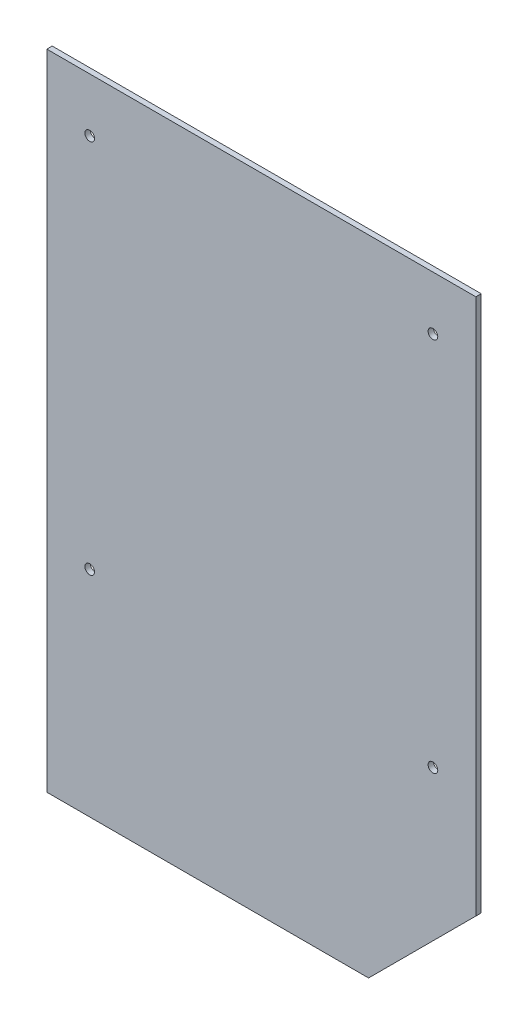
from build123d import *

# Parameters (mm, degrees)
SKETCH_1_W          = 400
SKETCH_1_H          = 600
EXTRUDE_1_DEPTH     = 5
SKETCH_2_R          = 4.5
CUT_EXTRUDE_1_DEPTH = 361.589794642
CHAMFER_1_SIZE      = 100


with BuildPart() as part:
    # 草图1 → 凸台-拉伸1 (new body)
    with BuildSketch(Plane.XY):
        Rectangle(SKETCH_1_W, SKETCH_1_H)
    extrude(amount=EXTRUDE_1_DEPTH)

    # 草图2 → 切除-拉伸1 (cut, through all)
    with BuildSketch(Plane.XY.offset(5)):
        with Locations((-160, 250)):
            Circle(SKETCH_2_R)
        with Locations((160, 250)):
            Circle(SKETCH_2_R)
        with Locations((160, -100)):
            Circle(SKETCH_2_R)
        with Locations((-160, -100)):
            Circle(SKETCH_2_R)
    extrude(amount=-CUT_EXTRUDE_1_DEPTH, mode=Mode.SUBTRACT)

    # 倒角1
    chamfer_1_edges = [part.edges().sort_by_distance(p)[0] for p in [
        (200, -300, 2.5),
    ]]
    chamfer(chamfer_1_edges, length=CHAMFER_1_SIZE)


solid = part.part
